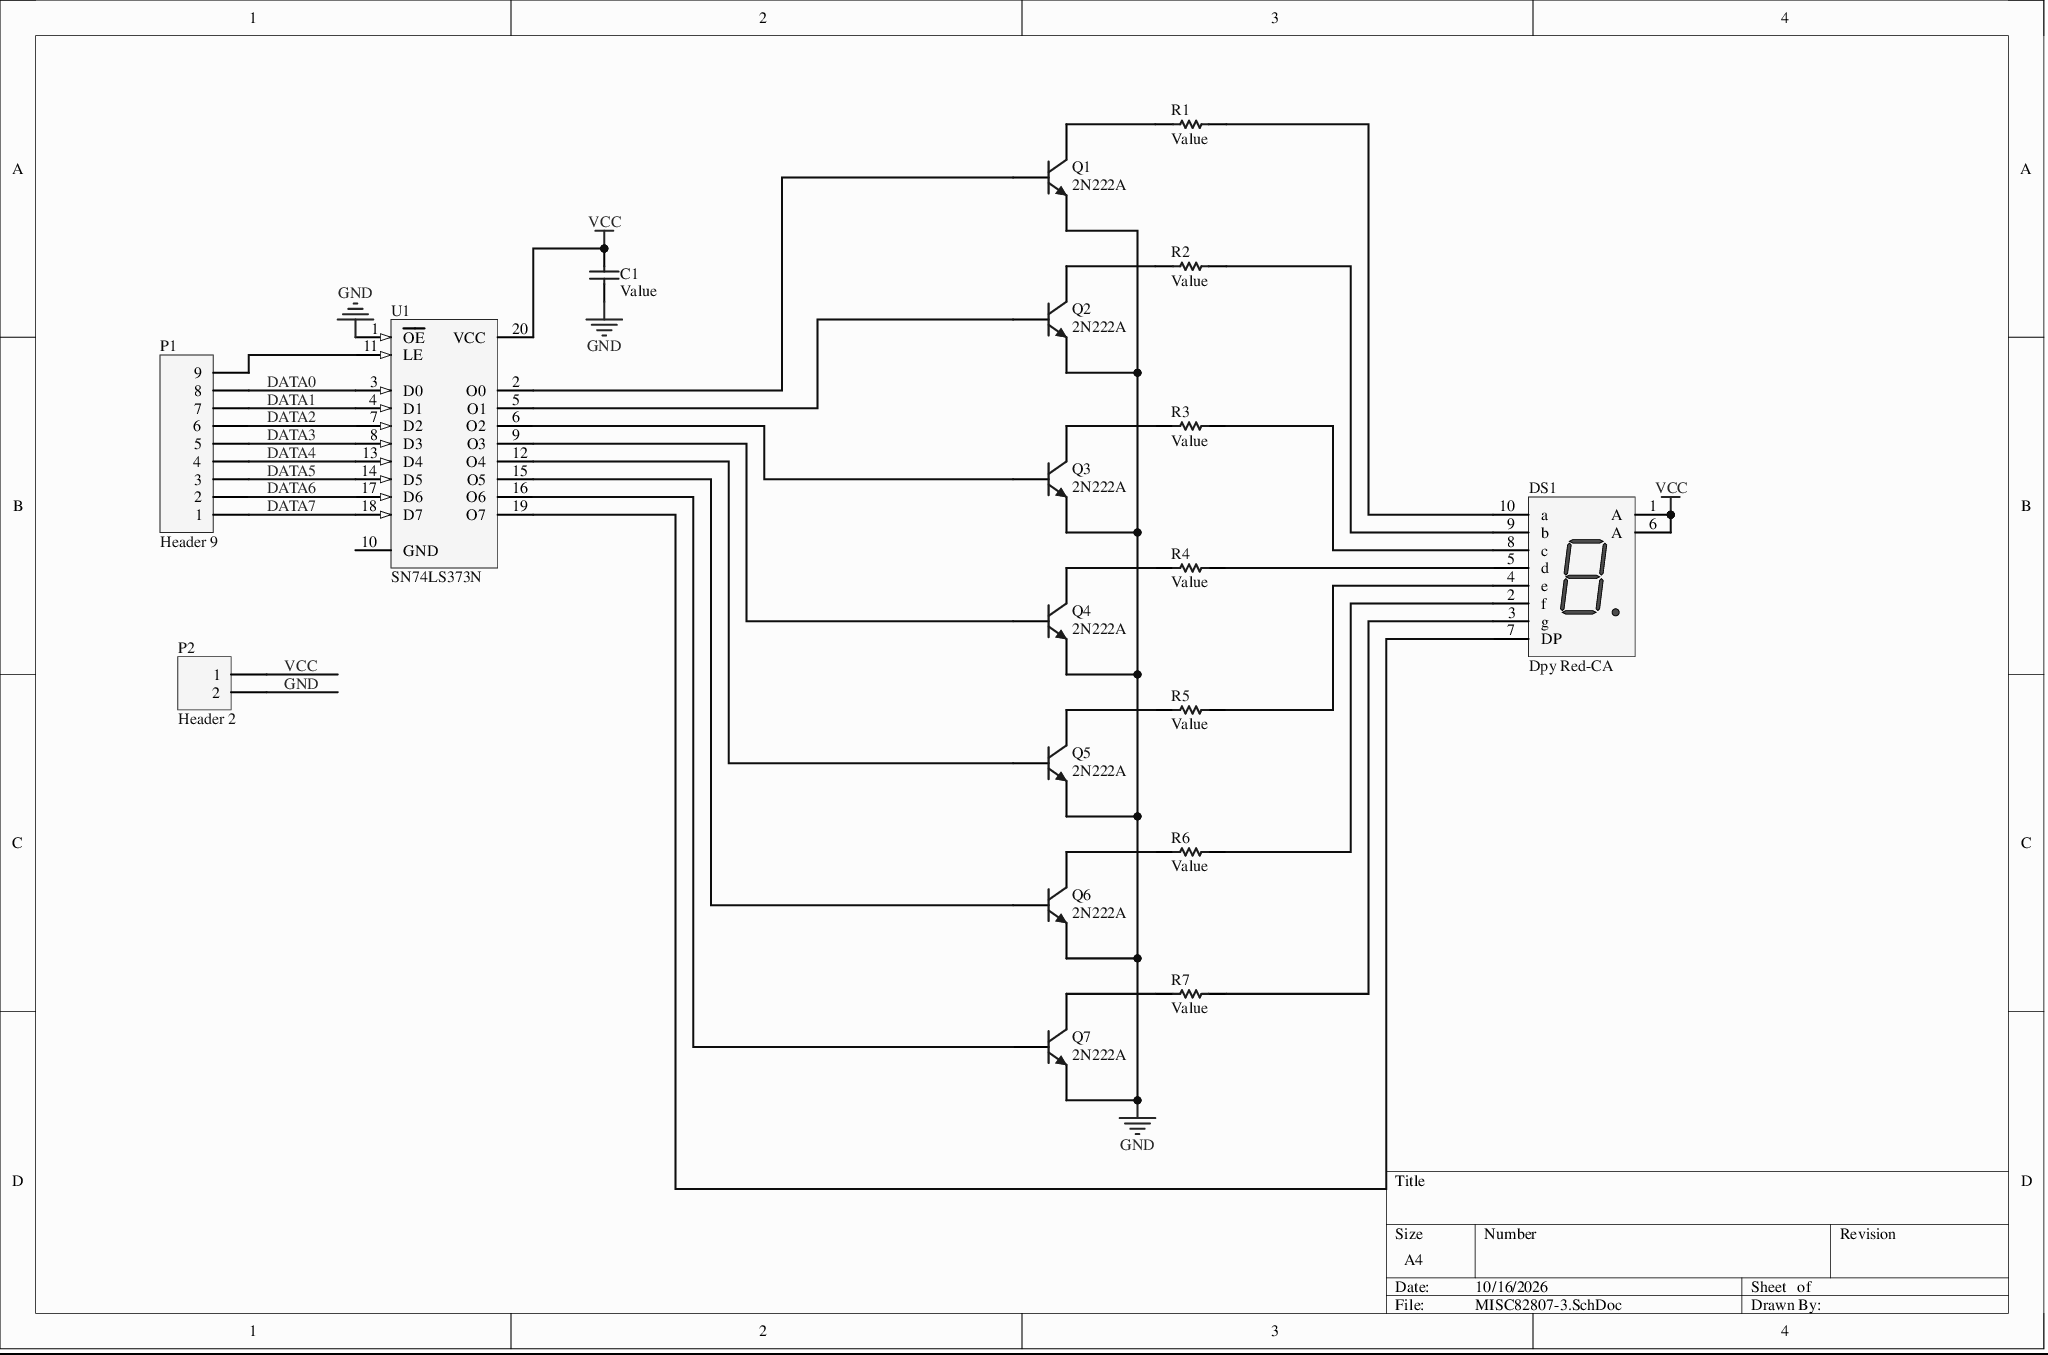
[diagram p0: MISC82807-3.SchDoc]
# Altium project MISC82807-7.PrjPcb
1 sheet, 19 parts. Net scope: global (net labels, ports and power ports of the same name join across sheets).
Board file: MISC82807-2.PcbDoc

## Sheet MISC82807-3.SchDoc
size A4

### Parts
C1  Value  [RAD-0.3]
DS1  Dpy Red-CA  [A]
P1  Header 9  [HDR1X9]
P2  Header 2  [HDR1X2]
Q1  2N222A  [TO-92A]
Q2  2N222A  [TO-92A]
Q3  2N222A  [TO-92A]
Q4  2N222A  [TO-92A]
Q5  2N222A  [TO-92A]
Q6  2N222A  [TO-92A]
Q7  2N222A  [TO-92A]
R1  Value  [AXIAL-0.3]
R2  Value  [AXIAL-0.3]
R3  Value  [AXIAL-0.3]
R4  Value  [AXIAL-0.3]
R5  Value  [AXIAL-0.3]
R6  Value  [AXIAL-0.3]
R7  Value  [AXIAL-0.3]
U1  SN74LS373N  [738-03]

### Nets
GND: C1.1 P2.2 Q1.1(E) Q2.1(E) Q3.1(E) Q4.1(E) Q5.1(E) Q6.1(E) Q7.1(E) U1.1(~{OE})
VCC: C1.2 DS1.1(A) DS1.6(A) P2.1 U1.20(VCC)
DATA0: P1.8 U1.3(D0)
DATA1: P1.7 U1.4(D1)
DATA2: P1.6 U1.7(D2)
DATA3: P1.5 U1.8(D3)
DATA4: P1.4 U1.13(D4)
DATA5: P1.3 U1.14(D5)
DATA6: P1.2 U1.17(D6)
DATA7: P1.1 U1.18(D7)
NetDS1_2: DS1.2(f) R6.2
NetDS1_3: DS1.3(g) R7.2
NetDS1_4: DS1.4(e) R5.2
NetDS1_5: DS1.5(d) R4.2
NetDS1_7: DS1.7(DP) U1.19(O7)
NetDS1_8: DS1.8(c) R3.2
NetDS1_9: DS1.9(b) R2.2
NetDS1_10: DS1.10(a) R1.2
NetP1_9: P1.9 U1.11(LE)
NetQ1_2: Q1.2(B) U1.2(O0)
NetQ1_3: Q1.3(C) R1.1
NetQ2_2: Q2.2(B) U1.5(O1)
NetQ2_3: Q2.3(C) R2.1
NetQ3_2: Q3.2(B) U1.6(O2)
NetQ3_3: Q3.3(C) R3.1
NetQ4_2: Q4.2(B) U1.9(O3)
NetQ4_3: Q4.3(C) R4.1
NetQ5_2: Q5.2(B) U1.12(O4)
NetQ5_3: Q5.3(C) R5.1
NetQ6_2: Q6.2(B) U1.15(O5)
NetQ6_3: Q6.3(C) R6.1
NetQ7_2: Q7.2(B) U1.16(O6)
NetQ7_3: Q7.3(C) R7.1

Not connected (* = marked no-connect by the designer): U1 10(GND)

### Library data of the parts
C1 = Cap: Capacitor; Value: 100pF; Published: 8-Jun-2000; LatestRevisionDate: 17-Jul-2002; LatestRevisionNote: Re-released for DXP Platform.; PackageReference: RAD-0.3; PackageDescription: Radial Cap, Thru-Hole; 2 Leads; 0.3 in Pin Spacing; Publisher: Altium Limited
DS1 = Dpy Red-CA: 7.62 mm Black Surface HER 7-Segment Display: CA, RH DP; MinimumIntensity: 360 ucd; Note: IF = 5 mA; Colour: High Efficiency Red (HER); Note: Pins 1 and 6 are redundant Anodes.; Published: 8-Jun-2000; LatestRevisionDate: 17-Dec-2003; LatestRevisionNote: Schematic revised, PCB Footprint replaced.; DatasheetVersion: 19-Feb-2002; PackageVersion: 11-Feb-2002; PackageReference: A; PackageDescription: LED, 7-Segment Display, 7.62 mm, RHD; 10 Leads; Row Space 5.08 mm; Pitch 2.54 mm; ComponentLink1Description: Manufacturer Link; Publisher: Altium Limited
P1 = Header 9: Header, 9-Pin; LatestRevisionDate: 17-Jul-2002; LatestRevisionNote: Re-released for DXP Platform.; Publisher: Altium Limited
P2 = Header 2: Header, 2-Pin; LatestRevisionDate: 17-Jul-2002; LatestRevisionNote: Re-released for DXP Platform.; Publisher: Altium Limited
Q1-Q7 = 2N3904: NPN General Purpose Amplifier; Published: 8-Jun-2000; LatestRevisionDate: 15-Jan-2003; LatestRevisionNote: PCB Footprint 'BCY-W3/D4.7' replaced; DatasheetVersion: 1997; PackageVersion: Sep-1998; PackageReference: TO-92A; PackageDescription: TO, Flat Index; 3 In-Line, Axial Leads; Body Dia. 4.5mm; Leads 0.51 x 0.48 mm (max); ComponentLink1Description: Manufacturer Link; ComponentLink2Description: Datasheet; ComponentLink2URL: http://www.fairchildsemi.com/ds/2N%2F2N3904.pdf; Publisher: Altium Limited
R1-R7 = Res1: Resistor; Value: 1K; Published: 8-Jun-2000; LatestRevisionDate: 17-Jul-2002; LatestRevisionNote: Re-released for DXP Platform.; PackageReference: AXIAL-0.3; PackageDescription: Axial Device, Thru-Hole; 2 Leads; 0.3 in Pin Spacing; Publisher: Altium Limited
U1 = SN74LS373N: Octal Transparent Latch with 3-State Outputs; Package Information: Latest Revision: 1996; Code - JEDEC: MS-001-AD; Published: 15-Apr-2002; Datasheet: Latest Revision: Dec-1999; Package Reference: 738-03; Publisher: Altium Limited